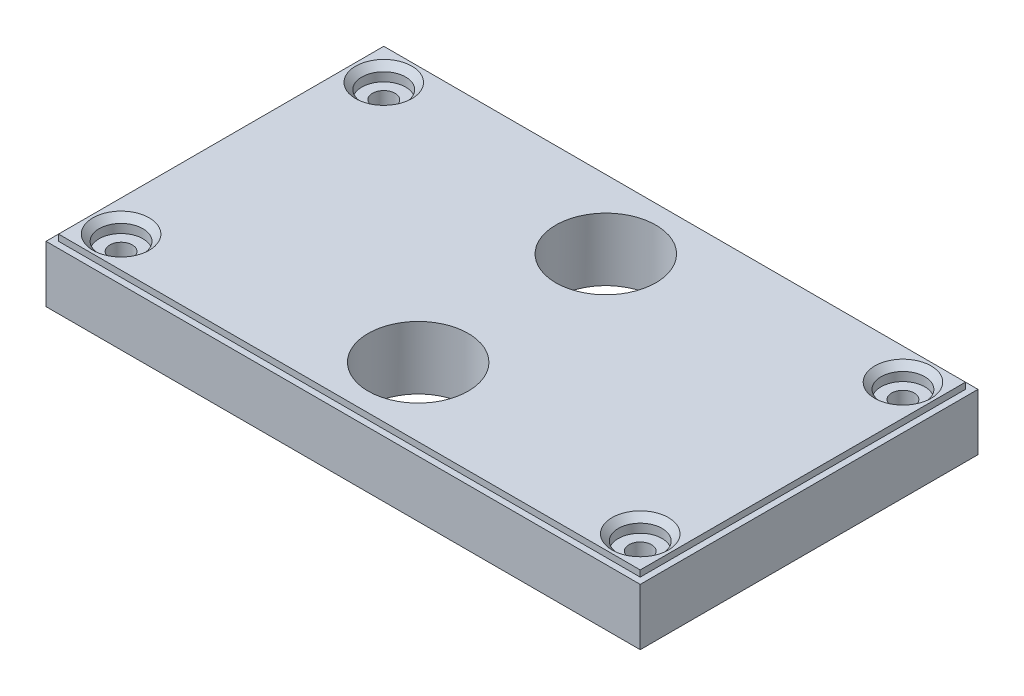
SolidWorks part; units mm, degrees
ref_plane "Front Plane" through (0, 0, 0) normal (0, 0, 1) x (1, 0, 0)
ref_plane "Top Plane" through (0, 0, 0) normal (0, 1, 0) x (1, 0, 0)
ref_plane "Right Plane" through (0, 0, 0) normal (1, 0, 0) x (0, 0, -1)
sketch "Sketch1" plane through (0, 0, 0) normal (0, 1, 0) x (1, 0, 0)
  line L1 (0, 0) -> (95, 0)
  line L2 (0, 0) -> (0, 54)
  line L3 (0, 54) -> (95, 54)
  line L4 (95, 0) -> (95, 54)
  dimension "D1" = 54
  dimension "D2" = 95
extrude "Boss-Extrude1" add sketch "Sketch1" along normal blind 10.05
sketch "Sketch2" plane through (0, 10.05, 0) normal (0, 1, 0) x (1, 0, 0)
  line L8 (1, 53) -> (1, 1)
  line L9 (1, 1) -> (94, 1)
  line L10 (94, 1) -> (94, 53)
  line L11 (94, 53) -> (1, 53)
  line L12 (1, 53) -> (1, 1)
  line L13 (1, 1) -> (94, 1)
  line L14 (94, 1) -> (94, 53)
  line L15 (94, 53) -> (1, 53)
  dimension "D1" = 1
extrude "Cut-Extrude1" cut sketch "Sketch2" against normal blind 1 flip side to cut
sketch "Sketch3" plane through (0, 10.05, 0) normal (0, 1, 0) x (1, 0, 0)
  line L0 (0, 54) -> (0, 0) construction
  line L1 (95, 54) -> (0, 54) construction
  line L2 (47.5, 54) -> (47.5, 0) construction
  line L3 (0, 0) -> (95, 0) construction
  line L4 (0, 27) -> (95, 27) construction
  line L5 (95, 0) -> (95, 54) construction
  point P0 (6, 48)
  point P14 (89, 48)
  point P16 (89, 6)
  point P17 (6, 6)
  dimension "D1" = 6
  dimension "D2" = 6
hole_wizard "CBORE for M3 Pan Head Screw1" positions "3DSketch1" profile "Sketch4" counterbore size "M3" standard "ISO" end condition up to next
sketch3d "3DSketch1"
  point P0 (6, 10.05, -48)
  point P3 (89, 10.05, -48)
  point P6 (89, 10.05, -6)
  point P9 (6, 10.05, -6)
sketch "Sketch4" plane through (6, 10.05, -48) normal (1, 0, 0) x (0, 0, 1)
  line L0 (0, 0) -> (0, 10.05)
  line L1 (0, 10.05) -> (1.8, 10.05)
  line L3 (1.8, 10.05) -> (1.8, 2.4)
  line L4 (1.8, 2.4) -> (3.5, 2.4)
  line L5 (3.5, 2.4) -> (3.5, 0)
  line L7 (3.5, 0) -> (0, 0)
  line L11 (0, -6.35) -> (0, 107.95) construction
  dimension "Thru Hole Dia." = 3.6
  dimension "Thru Hole Depth" = 10.05
  dimension "C'Bore Dia." = 7
  dimension "C'Bore Depth" = 2.4
chamfer "Chamfer1" distance 1 angle 45 4 edges at (89, 10.05, -2.5) (89, 10.05, -44.5) (6, 10.05, -2.5) (6, 10.05, -44.5)
sketch "Sketch5" plane through (0, 10.05, 0) normal (0, 1, 0) x (1, 0, 0)
  line L1 (47.5, 54) -> (47.5, 0) construction
  line L2 (95, 54) -> (0, 54) construction
  line L4 (0, 27) -> (95, 27) construction
  line L5 (0, 27) -> (95, 27)
  circle A0 centre (47.5, 42) radius 8
  circle A1 centre (47.5, 12) radius 8
  dimension "D1" = 12
  dimension "D2" = 16
extrude "Cut-Extrude2" cut sketch "Sketch5" against normal up to next contours A0 | A1
